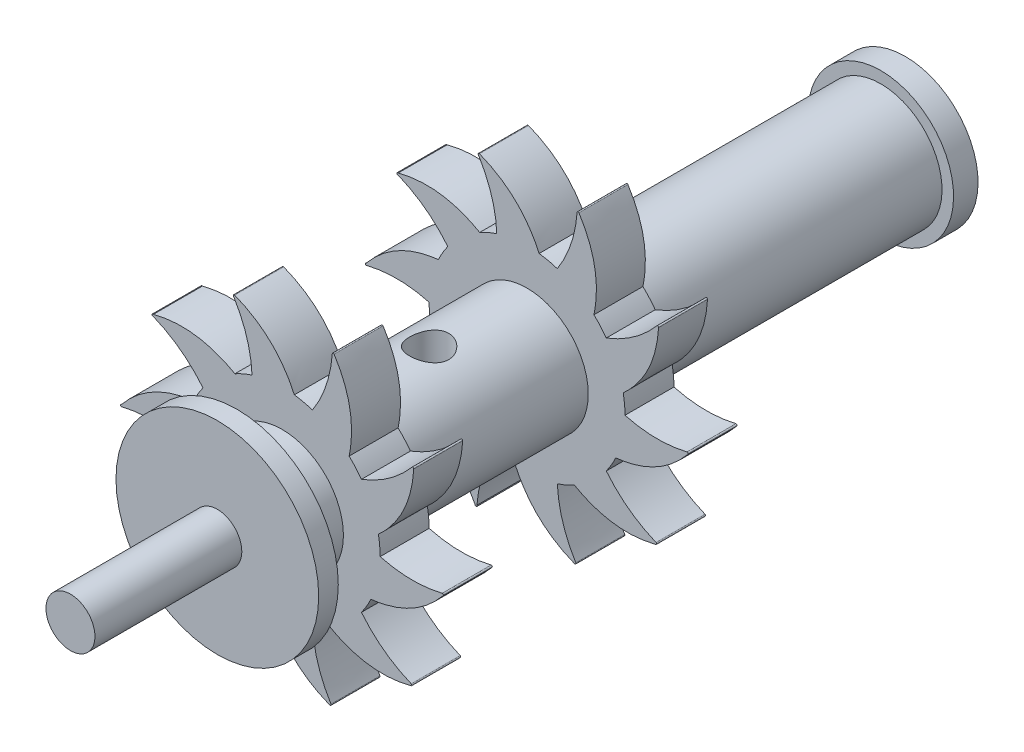
from build123d import *

# Parameters (mm, degrees)
SKETCH1_R               = 12.5
BOSS_EXTRUDE1_DEPTH     = 75
BOSS_EXTRUDE2_START     = 5
SKETCH2_R               = 14.854411906
SKETCH2_R_2             = 12.5
BOSS_EXTRUDE2_DEPTH     = 5
SKETCH3_R               = 12.5
BOSS_EXTRUDE3_DEPTH     = 40
SKETCH4_R               = 12.5
BOSS_EXTRUDE4_DEPTH     = 10
BOSS_EXTRUDE5_START     = 48
BOSS_EXTRUDE5_DEPTH     = 8
CUT_EXTRUDE1_DEPTH      = 41
CUT_EXTRUDE1_DEPTH_BACK = 34
SKETCH5_R               = 4
SKETCH7_R               = 15.333333333
CUT_EXTRUDE2_DEPTH      = 58
SKETCH8_R               = 20.7
BOSS_EXTRUDE6_DEPTH     = 4
SKETCH9_R               = 5
BOSS_EXTRUDE7_DEPTH     = 30


with BuildPart() as part:
    # Sketch1 → Boss-Extrude1 (new body)
    with BuildSketch(Plane.XY):
        Circle(SKETCH1_R)
    extrude(amount=BOSS_EXTRUDE1_DEPTH)

    # Sketch2 → Boss-Extrude2 (add)
    with BuildSketch(Plane(origin=(0, 0, 2.75), x_dir=(-1, 0, 0), z_dir=(0, 0, -1)).offset(BOSS_EXTRUDE2_START)):
        with Locations(Location((0, 0, 0), (0, 0, 90))):
            Circle(SKETCH2_R)
        with Locations(Location((0, 0, 0), (0, 0, 90))):
            Circle(SKETCH2_R_2, mode=Mode.SUBTRACT)
    extrude(amount=-BOSS_EXTRUDE2_DEPTH)

    # Sketch3 → Boss-Extrude3 (add)
    with BuildSketch(Plane.XY.offset(75)):
        with Locations(Location((0, 0, 0), (0, 0, 90))):
            Circle(SKETCH3_R)
    extrude(amount=BOSS_EXTRUDE3_DEPTH)

    # Sketch4 → Boss-Extrude4 (add)
    # profile 1 of 2: a face of its own
    with BuildSketch(Plane.XY.offset(115)):
        with BuildLine():
            add(Edge.make_bspline(
                [(26.862027902, 18.93904339), (26.507528375, 12.898307619), (24.087109777, 7.822641936), (19.638286439, 3.786516304)],
                knots=[0.031773445, 0.031773445, 0.031773445, 0.031773445, 1, 1, 1, 1], degree=3))
            ThreePointArc((19.638286439, 3.786516304), (19.909366248, 1.901876864), (20, 0))
            add(Edge.make_bspline(
                [(32.662279473, -0.145864864), (28.426225533, -1.170236967), (24.194058729, -1.121291137), (20, 0)],
                knots=[0.04334964, 0.04334964, 0.04334964, 0.04334964, 1, 1, 1, 1], degree=3))
            ThreePointArc((32.662279473, -0.145864864), (32.878680047, -0.2339289), (32.863927473, -0.467095888))
            add(Edge.make_bspline(
                [(32.863927473, -0.467095888), (29.026475932, -5.145784191), (24.084914719, -7.82939763), (18.113365911, -8.47973911)],
                knots=[0.031773445, 0.031773445, 0.031773445, 0.031773445, 1, 1, 1, 1], degree=3))
            ThreePointArc((18.113365911, -8.47973911), (17.224910814, -10.163781159), (16.180339887, -11.755705046))
            add(Edge.make_bspline(
                [(26.338601953, -19.316413334), (22.309451512, -17.655257741), (18.91432628, -15.1280545), (16.180339887, -11.755705046)],
                knots=[0.04334964, 0.04334964, 0.04334964, 0.04334964, 1, 1, 1, 1], degree=3))
            ThreePointArc((26.338601953, -19.316413334), (26.461910953, -19.514855702), (26.312923754, -19.694820413))
            add(Edge.make_bspline(
                [(26.312923754, -19.694820413), (20.458296257, -21.224361339), (14.883100854, -20.490873413), (9.669755255, -17.5070224)],
                knots=[0.031773445, 0.031773445, 0.031773445, 0.031773445, 1, 1, 1, 1], degree=3))
            ThreePointArc((9.669755255, -17.5070224), (7.961124902, -18.347220233), (6.180339887, -19.021130326))
            add(Edge.make_bspline(
                [(9.954473703, -31.108748452), (7.671225283, -27.396570137), (6.409964067, -23.356415227), (6.180339887, -19.021130326)],
                knots=[0.04334964, 0.04334964, 0.04334964, 0.04334964, 1, 1, 1, 1], degree=3))
            ThreePointArc((9.954473703, -31.108748452), (9.937591283, -31.341770911), (9.711277503, -31.399792942))
            add(Edge.make_bspline(
                [(9.711277503, -31.399792942), (4.075742764, -29.195953845), (-0.003551679, -25.325532011), (-2.467373245, -19.847218175)],
                knots=[0.031773445, 0.031773445, 0.031773445, 0.031773445, 1, 1, 1, 1], degree=3))
            ThreePointArc((-2.467373245, -19.847218175), (-4.343540133, -19.522644778), (-6.180339887, -19.021130326))
            add(Edge.make_bspline(
                [(-10.231925161, -31.018599008), (-9.897148269, -26.673323917), (-8.542786553, -22.663419192), (-6.180339887, -19.021130326)],
                knots=[0.04334964, 0.04334964, 0.04334964, 0.04334964, 1, 1, 1, 1], degree=3))
            ThreePointArc((-10.231925161, -31.018599008), (-10.351553903, -31.320434197), (-10.599746679, -31.111111807))
            add(Edge.make_bspline(
                [(-10.599746679, -31.111111807), (-13.863605936, -26.015684316), (-14.888847591, -20.486698164), (-13.662049029, -14.606451189)],
                knots=[0.031773445, 0.031773445, 0.031773445, 0.031773445, 1, 1, 1, 1], degree=3))
            ThreePointArc((-13.662049029, -14.606451189), (-14.98912047, -13.241082567), (-16.180339887, -11.755705046))
            add(Edge.make_bspline(
                [(-26.510076384, -19.080399027), (-23.685147573, -15.761774553), (-20.232483069, -13.313767328), (-16.180339887, -11.755705046)],
                knots=[0.04334964, 0.04334964, 0.04334964, 0.04334964, 1, 1, 1, 1], degree=3))
            ThreePointArc((-26.510076384, -19.080399027), (-26.784272342, -19.254272814), (-26.862027902, -18.93904339))
            add(Edge.make_bspline(
                [(-26.862027902, -18.93904339), (-26.507528375, -12.898307619), (-24.087109777, -7.822641936), (-19.638286439, -3.786516304)],
                knots=[0.031773445, 0.031773445, 0.031773445, 0.031773445, 1, 1, 1, 1], degree=3))
            ThreePointArc((-19.638286439, -3.786516304), (-19.909366248, -1.901876864), (-20, 0))
            add(Edge.make_bspline(
                [(-32.662279473, 0.145864864), (-28.426225533, 1.170236967), (-24.194058729, 1.121291137), (-20, 0)],
                knots=[0.04334964, 0.04334964, 0.04334964, 0.04334964, 1, 1, 1, 1], degree=3))
            ThreePointArc((-32.662279473, 0.145864864), (-32.986309111, 0.166366355), (-32.863927473, 0.467095888))
            add(Edge.make_bspline(
                [(-32.863927473, 0.467095888), (-29.026475932, 5.145784191), (-24.084914719, 7.82939763), (-18.113365911, 8.47973911)],
                knots=[0.031773445, 0.031773445, 0.031773445, 0.031773445, 1, 1, 1, 1], degree=3))
            ThreePointArc((-18.113365911, 8.47973911), (-17.224910814, 10.163781159), (-16.180339887, 11.755705046))
            add(Edge.make_bspline(
                [(-26.338601953, 19.316413334), (-22.309451512, 17.655257741), (-18.91432628, 15.1280545), (-16.180339887, 11.755705046)],
                knots=[0.04334964, 0.04334964, 0.04334964, 0.04334964, 1, 1, 1, 1], degree=3))
            ThreePointArc((-26.338601953, 19.316413334), (-26.588696962, 19.523459231), (-26.312923754, 19.694820413))
            add(Edge.make_bspline(
                [(-26.312923754, 19.694820413), (-20.458296257, 21.224361339), (-14.883100854, 20.490873413), (-9.669755255, 17.5070224)],
                knots=[0.031773445, 0.031773445, 0.031773445, 0.031773445, 1, 1, 1, 1], degree=3))
            ThreePointArc((-9.669755255, 17.5070224), (-7.961124902, 18.347220233), (-6.180339887, 19.021130326))
            add(Edge.make_bspline(
                [(-9.954473703, 31.108748452), (-7.671225283, 27.396570137), (-6.336636381, 23.383531358), (-6.180339887, 19.021130326)],
                knots=[0.04334964, 0.04334964, 0.04334964, 0.04334964, 1, 1, 1, 1], degree=3))
            ThreePointArc((-9.954473703, 31.108748452), (-9.937591283, 31.341770911), (-9.711277503, 31.399792942))
            add(Edge.make_bspline(
                [(-9.711277503, 31.399792942), (-4.075742764, 29.195953845), (0.003551679, 25.325532011), (2.467373245, 19.847218175)],
                knots=[0.031773445, 0.031773445, 0.031773445, 0.031773445, 1, 1, 1, 1], degree=3))
            ThreePointArc((2.467373245, 19.847218175), (4.343540133, 19.522644778), (6.180339887, 19.021130326))
            add(Edge.make_bspline(
                [(10.231925161, 31.018599008), (9.897148269, 26.673323917), (8.542786553, 22.663419192), (6.180339887, 19.021130326)],
                knots=[0.04334964, 0.04334964, 0.04334964, 0.04334964, 1, 1, 1, 1], degree=3))
            ThreePointArc((10.231925161, 31.018599008), (10.382550492, 31.1971949), (10.599746679, 31.111111807))
            add(Edge.make_bspline(
                [(10.599746679, 31.111111807), (13.863605936, 26.015684316), (14.888847591, 20.486698164), (13.662049029, 14.606451189)],
                knots=[0.031773445, 0.031773445, 0.031773445, 0.031773445, 1, 1, 1, 1], degree=3))
            ThreePointArc((13.662049029, 14.606451189), (14.98912047, 13.241082567), (16.180339887, 11.755705046))
            add(Edge.make_bspline(
                [(26.510076384, 19.080399027), (23.685147573, 15.761774553), (20.232483069, 13.313767328), (16.180339887, 11.755705046)],
                knots=[0.04334964, 0.04334964, 0.04334964, 0.04334964, 1, 1, 1, 1], degree=3))
            ThreePointArc((26.510076384, 19.080399027), (26.736910868, 19.136350791), (26.862027902, 18.93904339))
        make_face()
        with Locations(Location((0, 0, 0), (0, 0, 90))):
            Circle(SKETCH4_R, mode=Mode.SUBTRACT)
    # profile 2 of 2: a face of its own
    with BuildSketch(Plane.XY.offset(115)):
        with Locations(Location((0, 0, 0), (0, 0, 90))):
            Circle(SKETCH4_R)
    extrude(amount=BOSS_EXTRUDE4_DEPTH)

    # Sketch6 → Boss-Extrude5 (add)
    with BuildSketch(Plane(origin=(0, 0, 115), x_dir=(-1, 0, 0), z_dir=(0, 0, -1)).offset(BOSS_EXTRUDE5_START)):
        with BuildLine():
            ThreePointArc((-19.638286439, 3.786516304), (-19.909366248, 1.901876864), (-20, 0))
            add(Edge.make_bspline(
                [(-20, 0), (-24.194058729, -1.121291137), (-28.426225533, -1.170236967), (-32.662279473, -0.145864864)],
                knots=[0.04334964, 0.04334964, 0.04334964, 0.04334964, 1, 1, 1, 1], degree=3))
            ThreePointArc((-32.662279473, -0.145864864), (-32.878680047, -0.2339289), (-32.863927473, -0.467095888))
            add(Edge.make_bspline(
                [(-32.863927473, -0.467095888), (-29.026475932, -5.145784191), (-24.084914719, -7.82939763), (-18.113365911, -8.47973911)],
                knots=[0.031773445, 0.031773445, 0.031773445, 0.031773445, 1, 1, 1, 1], degree=3))
            ThreePointArc((-18.113365911, -8.47973911), (-17.224910814, -10.163781159), (-16.180339887, -11.755705046))
            add(Edge.make_bspline(
                [(-16.180339887, -11.755705046), (-18.91432628, -15.1280545), (-22.309451512, -17.655257741), (-26.338601953, -19.316413334)],
                knots=[0.04334964, 0.04334964, 0.04334964, 0.04334964, 1, 1, 1, 1], degree=3))
            ThreePointArc((-26.338601953, -19.316413334), (-26.461910953, -19.514855702), (-26.312923754, -19.694820413))
            add(Edge.make_bspline(
                [(-26.312923754, -19.694820413), (-20.458296257, -21.224361339), (-14.883100854, -20.490873413), (-9.669755255, -17.5070224)],
                knots=[0.031773445, 0.031773445, 0.031773445, 0.031773445, 1, 1, 1, 1], degree=3))
            ThreePointArc((-9.669755255, -17.5070224), (-7.961124902, -18.347220233), (-6.180339887, -19.021130326))
            add(Edge.make_bspline(
                [(-6.180339887, -19.021130326), (-6.409964067, -23.356415227), (-7.671225283, -27.396570137), (-9.954473703, -31.108748452)],
                knots=[0.04334964, 0.04334964, 0.04334964, 0.04334964, 1, 1, 1, 1], degree=3))
            ThreePointArc((-9.954473703, -31.108748452), (-9.937591283, -31.341770911), (-9.711277503, -31.399792942))
            add(Edge.make_bspline(
                [(-9.711277503, -31.399792942), (-4.075742764, -29.195953845), (0.003551679, -25.325532011), (2.467373245, -19.847218175)],
                knots=[0.031773445, 0.031773445, 0.031773445, 0.031773445, 1, 1, 1, 1], degree=3))
            ThreePointArc((2.467373245, -19.847218175), (4.343540133, -19.522644778), (6.180339887, -19.021130326))
            add(Edge.make_bspline(
                [(6.180339887, -19.021130326), (8.542786553, -22.663419192), (9.897148269, -26.673323917), (10.231925161, -31.018599008)],
                knots=[0.04334964, 0.04334964, 0.04334964, 0.04334964, 1, 1, 1, 1], degree=3))
            ThreePointArc((10.231925161, -31.018599008), (10.351553903, -31.320434197), (10.599746679, -31.111111807))
            add(Edge.make_bspline(
                [(10.599746679, -31.111111807), (13.863605936, -26.015684316), (14.888847591, -20.486698164), (13.662049029, -14.606451189)],
                knots=[0.031773445, 0.031773445, 0.031773445, 0.031773445, 1, 1, 1, 1], degree=3))
            ThreePointArc((13.662049029, -14.606451189), (14.98912047, -13.241082567), (16.180339887, -11.755705046))
            add(Edge.make_bspline(
                [(16.180339887, -11.755705046), (20.232483069, -13.313767328), (23.685147573, -15.761774553), (26.510076384, -19.080399027)],
                knots=[0.04334964, 0.04334964, 0.04334964, 0.04334964, 1, 1, 1, 1], degree=3))
            ThreePointArc((26.510076384, -19.080399027), (26.784272342, -19.254272814), (26.862027902, -18.93904339))
            add(Edge.make_bspline(
                [(26.862027902, -18.93904339), (26.507528375, -12.898307619), (24.087109777, -7.822641936), (19.638286439, -3.786516304)],
                knots=[0.031773445, 0.031773445, 0.031773445, 0.031773445, 1, 1, 1, 1], degree=3))
            ThreePointArc((19.638286439, -3.786516304), (19.909366248, -1.901876864), (20, 0))
            add(Edge.make_bspline(
                [(20, 0), (24.194058729, 1.121291137), (28.426225533, 1.170236967), (32.662279473, 0.145864864)],
                knots=[0.04334964, 0.04334964, 0.04334964, 0.04334964, 1, 1, 1, 1], degree=3))
            ThreePointArc((32.662279473, 0.145864864), (32.986309111, 0.166366355), (32.863927473, 0.467095888))
            add(Edge.make_bspline(
                [(32.863927473, 0.467095888), (29.026475932, 5.145784191), (24.084914719, 7.82939763), (18.113365911, 8.47973911)],
                knots=[0.031773445, 0.031773445, 0.031773445, 0.031773445, 1, 1, 1, 1], degree=3))
            ThreePointArc((18.113365911, 8.47973911), (17.224910814, 10.163781159), (16.180339887, 11.755705046))
            add(Edge.make_bspline(
                [(16.180339887, 11.755705046), (18.91432628, 15.1280545), (22.309451512, 17.655257741), (26.338601953, 19.316413334)],
                knots=[0.04334964, 0.04334964, 0.04334964, 0.04334964, 1, 1, 1, 1], degree=3))
            ThreePointArc((26.338601953, 19.316413334), (26.588696962, 19.523459231), (26.312923754, 19.694820413))
            add(Edge.make_bspline(
                [(26.312923754, 19.694820413), (20.458296257, 21.224361339), (14.883100854, 20.490873413), (9.669755255, 17.5070224)],
                knots=[0.031773445, 0.031773445, 0.031773445, 0.031773445, 1, 1, 1, 1], degree=3))
            ThreePointArc((9.669755255, 17.5070224), (7.961124902, 18.347220233), (6.180339887, 19.021130326))
            add(Edge.make_bspline(
                [(6.180339887, 19.021130326), (6.336636381, 23.383531358), (7.671225283, 27.396570137), (9.954473703, 31.108748452)],
                knots=[0.04334964, 0.04334964, 0.04334964, 0.04334964, 1, 1, 1, 1], degree=3))
            ThreePointArc((9.954473703, 31.108748452), (9.937591283, 31.341770911), (9.711277503, 31.399792942))
            add(Edge.make_bspline(
                [(9.711277503, 31.399792942), (4.075742764, 29.195953845), (-0.003551679, 25.325532011), (-2.467373245, 19.847218175)],
                knots=[0.031773445, 0.031773445, 0.031773445, 0.031773445, 1, 1, 1, 1], degree=3))
            ThreePointArc((-2.467373245, 19.847218175), (-4.343540133, 19.522644778), (-6.180339887, 19.021130326))
            add(Edge.make_bspline(
                [(-6.180339887, 19.021130326), (-8.542786553, 22.663419192), (-9.897148269, 26.673323917), (-10.231925161, 31.018599008)],
                knots=[0.04334964, 0.04334964, 0.04334964, 0.04334964, 1, 1, 1, 1], degree=3))
            ThreePointArc((-10.231925161, 31.018599008), (-10.382550492, 31.1971949), (-10.599746679, 31.111111807))
            add(Edge.make_bspline(
                [(-10.599746679, 31.111111807), (-13.863605936, 26.015684316), (-14.888847591, 20.486698164), (-13.662049029, 14.606451189)],
                knots=[0.031773445, 0.031773445, 0.031773445, 0.031773445, 1, 1, 1, 1], degree=3))
            ThreePointArc((-13.662049029, 14.606451189), (-14.98912047, 13.241082567), (-16.180339887, 11.755705046))
            add(Edge.make_bspline(
                [(-16.180339887, 11.755705046), (-20.232483069, 13.313767328), (-23.685147573, 15.761774553), (-26.510076384, 19.080399027)],
                knots=[0.04334964, 0.04334964, 0.04334964, 0.04334964, 1, 1, 1, 1], degree=3))
            ThreePointArc((-26.510076384, 19.080399027), (-26.736910868, 19.136350791), (-26.862027902, 18.93904339))
            add(Edge.make_bspline(
                [(-26.862027902, 18.93904339), (-26.507528375, 12.898307619), (-24.087109777, 7.822641936), (-19.638286439, 3.786516304)],
                knots=[0.031773445, 0.031773445, 0.031773445, 0.031773445, 1, 1, 1, 1], degree=3))
        make_face()
    extrude(amount=-BOSS_EXTRUDE5_DEPTH)

    # Sketch5 → Cut-Extrude1 (cut, two sides: drawn at the far end of the back side and taken through both)
    with BuildSketch(Plane(origin=(0, 0, 0), x_dir=(1, 0, 0), z_dir=(0, 1, 0)).offset(-CUT_EXTRUDE1_DEPTH_BACK)):
        with Locations(Location((0, -95, 0), (0, 0, 90))):
            Circle(SKETCH5_R)
    extrude(amount=CUT_EXTRUDE1_DEPTH + CUT_EXTRUDE1_DEPTH_BACK, mode=Mode.SUBTRACT)

    # Mirror1: part across plane


with BuildPart() as part_1:
    add(part.part)
    add(part.part.mirror(Plane(origin=(0, 0, 95), x_dir=(1, 0, 0), z_dir=(0, 0, -1))))

    # Sketch7 → Cut-Extrude2 (cut)
    with BuildSketch(Plane.XY.offset(192.25)):
        Circle(SKETCH7_R)
    extrude(amount=-CUT_EXTRUDE2_DEPTH, mode=Mode.SUBTRACT)

    # Sketch8 → Boss-Extrude6 (add)
    with BuildSketch(Plane.XY.offset(134.25)):
        Circle(SKETCH8_R)
    extrude(amount=BOSS_EXTRUDE6_DEPTH)

    # Sketch9 → Boss-Extrude7 (add)
    with BuildSketch(Plane.XY.offset(138.25)):
        Circle(SKETCH9_R)
    extrude(amount=BOSS_EXTRUDE7_DEPTH)


solid = part_1.part
